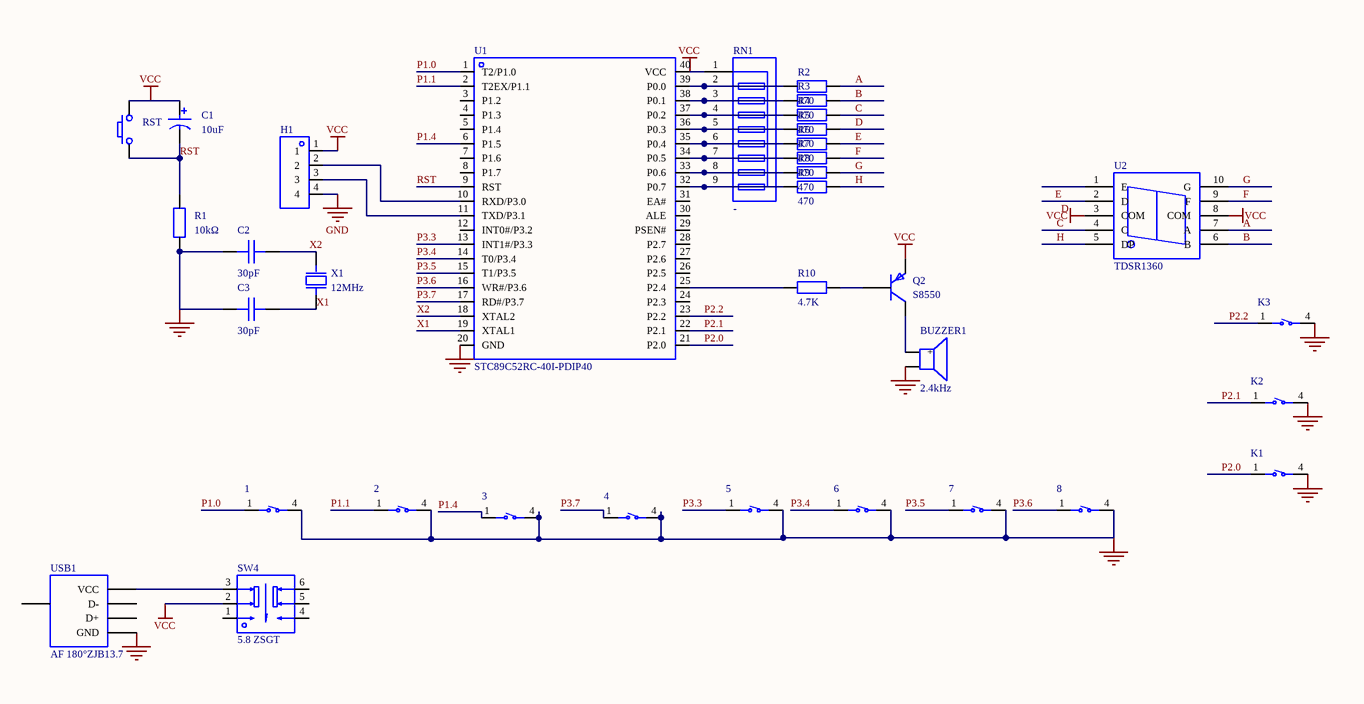
[diagram p0: MISC49928-3.schdoc]
# Altium project MISC49928-2.PrjPcb
1 sheet, 34 parts. Net scope: global (net labels, ports and power ports of the same name join across sheets).
Board file: MISC49928.pcbdoc

## Sheet MISC49928-3.schdoc
size 1187 x 839 mm; Version: V1.0; @Project Name: MISC49928; @Update Date: 2026-05-11; @Create Date: 2026-05-11; @Board Name: MISC49928; @Create Time: 23:58:54; @Page Count: 1; @Page No: 1; @Schematic Name: MISC49928; @Update Time: 23:58:54; Size: A4

### Parts
1  TS665CJ  [SW-TH_4P-L6.0-W6.0-P4.50-LS6.5]  (value not drawn)
2  TS665CJ  [SW-TH_4P-L6.0-W6.0-P4.50-LS6.5]  (value not drawn)
3  TS665CJ  [SW-TH_4P-L6.0-W6.0-P4.50-LS6.5]  (value not drawn)
4  TS665CJ  [SW-TH_4P-L6.0-W6.0-P4.50-LS6.5]  (value not drawn)
5  TS665CJ  [SW-TH_4P-L6.0-W6.0-P4.50-LS6.5]  (value not drawn)
6  TS665CJ  [SW-TH_4P-L6.0-W6.0-P4.50-LS6.5]  (value not drawn)
7  TS665CJ  [SW-TH_4P-L6.0-W6.0-P4.50-LS6.5]  (value not drawn)
8  TS665CJ  [SW-TH_4P-L6.0-W6.0-P4.50-LS6.5]  (value not drawn)
BUZZER1  2.4kHz  [BUZ-TH_BD12.0-P7.60-D0.6-FD]
C1  10uF  [CAP-TH_BD8.0-P3.50-D0.6-FD]
C2  30pF  [CAP-TH_L8.5-W5.0-P5.00-D1.2]
C3  30pF  [CAP-TH_L8.5-W5.0-P5.00-D1.2]
H1  (no value)  [HDR-TH_4P-P2.54-V-F]
K1  TS665CJ  [SW-TH_4P-L6.0-W6.0-P4.50-LS6.5]  (value not drawn)
K2  TS665CJ  [SW-TH_4P-L6.0-W6.0-P4.50-LS6.5]  (value not drawn)
K3  TS665CJ  [SW-TH_4P-L6.0-W6.0-P4.50-LS6.5]  (value not drawn)
Q2  S8550  [TO-92-3_L4.5-W3.5-P1.27-L]
R1  10kΩ  [RES-TH_BD2.4-L6.3-P10.30-D0.6]
R2  470  [R0603]
R3  470  [R0603]
R4  470  [R0603]
R5  470  [R0603]
R6  470  [R0603]
R7  470  [R0603]
R8  470  [R0603]
R9  470  [R0603]
R10  4.7K  [RES-TH_BD2.2-L6.5-P10.50-D0.6]
RN1  -  [RES-ARRAY-TH_9P-P2.54-D1.0]
RST  (no value)  [Key_TH_3.5x6x4.3]
SW4  5.8 ZSGT  [SW-TH_5.8ZSGT]
U1  STC89C52RC-40I-PDIP40  [DIP-40_L52.0-W13.7-P2.54-LS15.2-BL]
U2  TDSR1360  [LED-SEG-TH_10P-L17.6-W12.4-P2.54-S15.24-BL]
USB1  AF 180°ZJB13.7  [USB-A-TH_AF-ZJB13.7]
X1  12MHz  [HC-49US_L11.5-W4.5-P4.88]

### Nets
GND: 1.4(D) 2.4(D) 3.4(D) 4.4(D) 5.4(D) 6.4(D) 7.4(D) 8.4(D) BUZZER1.2 C2.1 C3.1 H1.4 K1.4(D) K2.4(D) K3.4(D) R1.1 U1.20(GND) USB1.4(GND)
VCC: C1.1 H1.1 Q2.1(E) RN1.1 RST.B SW4.2 U1.40(VCC) U2.3(COM) U2.8(COM)
A: R2.2 U2.7(A)
B: R3.2 U2.6(B)
C: R4.2 U2.4(C)
D: R5.2 U2.2(D)
E: R6.2 U2.1(E)
F: R7.2 U2.9(F)
G: R8.2 U2.10(G)
H: R9.2 U2.5(DP)
P1.0: 1.1(A) U1.1(T2/P1.0)
P1.1: 2.1(A) U1.2(T2EX/P1.1)
P1.4: 3.1(A) U1.6(P1.5)
P2.0: K1.1(A) U1.21(P2.0)
P2.1: K2.1(A) U1.22(P2.1)
P2.2: K3.1(A) U1.23(P2.2)
P3.3: 5.1(A) U1.13(INT1#/P3.3)
P3.4: 6.1(A) U1.14(T0/P3.4)
P3.5: 7.1(A) U1.15(T1/P3.5)
P3.6: 8.1(A) U1.16(WR#/P3.6)
P3.7: 4.1(A) U1.17(RD#/P3.7)
RST: C1.2 R1.2 RST.A U1.9(RST)
X1: C3.2 U1.19(XTAL1) X1.2(OSC2)
X2: C2.2 U1.18(XTAL2) X1.1(OSC1)
NetBUZZER1_1: BUZZER1.1(+) Q2.3(C)
NetH1_2: H1.2 U1.10(RXD/P3.0)
NetH1_3: H1.3 U1.11(TXD/P3.1)
NetQ2_2: Q2.2(B) R10.2
NetR2_1: R2.1 RN1.2 U1.39(P0.0)
NetR3_1: R3.1 RN1.3 U1.38(P0.1)
NetR4_1: R4.1 RN1.4 U1.37(P0.2)
NetR5_1: R5.1 RN1.5 U1.36(P0.3)
NetR6_1: R6.1 RN1.6 U1.35(P0.4)
NetR7_1: R7.1 RN1.7 U1.34(P0.5)
NetR8_1: R8.1 RN1.8 U1.33(P0.6)
NetR9_1: R9.1 RN1.9 U1.32(P0.7)
NetR10_1: R10.1 U1.25(P2.4)
NetSW4_3: SW4.3 USB1.1(VCC)

Not connected (* = marked no-connect by the designer): SW4 1 4 5 6; U1 3(P1.2) 4(P1.3) 5(P1.4) 7(P1.6) 8(P1.7) 12(INT0#/P3.2) 24(P2.3) 26(P2.5) 27(P2.6) 28(P2.7) 29(PSEN#) 30(ALE) 31(EA#); USB1 2(D-) 3(D+) 5(SHLD)

### Library data of the parts
1-8 K1-K3 = TS665CJ: Circuit structure: SPST; button shape: round button; actuating force: 2.5N; mounting: through-hole; switch length: 6mm; switch width: 6mm; switch height: 5mm; with bracket: no bracket; contact current: 50mA; rated voltage: 12V; with lamp: none; operating life: 5 ten-thousand cycles;; Manufacturer: SHOU HAN(首韩); AddInBom: yes; ModelId: 20eee248bc684ccd8cbdbb1d0d91ec6f0819f05c4eef4c71ace90d822a990e87; ModelName: SW-TH_4P-L6.0-W6.0-H5.0-LS6.5-P4.50; ModelTransform: 236.22,323.03,0,90,0,0,0,0,-137.795; Actuator/Cap Color: Black; Symbol: TS665CJ; Device: TS665CJ; LCSC Part Name: 6*6*5mm 直插 轻触开关; SupplierPart: C393938; ManufacturerPart: TS665CJ; Supplier Footprint: 插件-4P,6x6mm; JLCPCB Part Class: Extended Part; Datasheet: https://example.com/datasheet/TS665CJ/372550.html; Supplier: LCSC; ConvertToPcb: yes; FootprintName: SW-TH_4P-L6.0-W6.0-P4.50-LS6.5; Circuit: SPST; Actuator Style: Round button; Operating Force: 2.5N; Mounting Type: Through-hole; Length: 6mm; Width: 6mm; Switch Height: 5mm; with Bracket: No bracket; Contact Current: 50mA; Voltage Rating: 12V; With Lamp: None; Termination Style: PC pin; Life: 5 ten-thousand cycles; Operating Temperature: -25℃~+70℃
BUZZER1 = TMB12A05_C96093: Drive mode: active (built-in driver circuit); construction type: electromagnetic; rated voltage: 5V; frequency: 2.4kHz; sound pressure level (SPL): 85dB;; Manufacturer: 华能; AddInBom: yes; ModelId: 16ab50e14c5b4f2c986c135bdba60e370819f05c4eef4c71ace90d822a990e87; ModelName: BUZ-TH_D12.0-H9.5-P7.60; ModelTransform: 472.44,472.176,0,90,0,0,-0.787,0,-177.165; Voltage - Supply: 4V~8V; Current Consumption: 30mA; Symbol: TMB12A05; Device: TMB12A05_C96093; LCSC Part Name: 有源(内含驱动线路) 电磁式 2.4kHz; SupplierPart: C96093; ManufacturerPart: TMB12A05; Supplier Footprint: 插件,D=12mm; JLCPCB Part Class: Extended Part; Datasheet: https://example.com/datasheet/TMB12A05/97297.html; Supplier: LCSC; ConvertToPcb: yes; FootprintName: BUZ-TH_BD12.0-P7.60-D0.6-FD; Driver Circuitry: Active (built-in driver circuit); Technology: Electromagnetic; Voltage Rating: 5V; Value: 2.4kHz; Sound Pressure Level(SPL): 85dB; Diameter(φD): 12mm; Length: -; Width: -; Height: 9.8mm; Operating Temperature: -40℃~+85℃
C1 = ERK2GM100F12OT: Capacitance: 10uF; tolerance: ±20%; rated voltage: 400V; ripple current: 160mA@100kHz; equivalent series resistance (ESR): -;; Manufacturer: AISHI(艾华集团); AddInBom: yes; ModelId: a2c936ec27754f809f3966430e36f7670819f05c4eef4c71ace90d822a990e87; ModelName: CAP-TH_D8.0-H8.0-P3.50; ModelTransform: 314.96,314.862,0,180,0,0,0,0,-137.795; Pin Spacing: 3.5mm; Lifetime: 2000hrs@105℃; Symbol: ERK2GM100F12OT; Device: ERK2GM100F12OT; LCSC Part Name: 10uF ±20% 400V CLEAR 专门用于充电器; SupplierPart: C112497; ManufacturerPart: ERK2GM100F12OT; Supplier Footprint: 插件,D8xL12mm; JLCPCB Part Class: Extended Part; Datasheet: https://example.com/datasheet/ERK2GM100F12OT/113730.html; Supplier: LCSC; ConvertToPcb: yes; FootprintName: CAP-TH_BD8.0-P3.50-D0.6-FD; Value: 10uF; Tolerance: ±20%; Voltage Rating: 400V; Ripple Current: 160mA@100kHz; Equivalent Series Resistance(ESR): -; Diameter: 8mm; Height - Seated (Max): 12mm
C2 C3 = CC4-0805N300J500F3: Capacitance: 30pF; tolerance: ±5%; rated voltage: 50V; temperature coefficient: C0G;; Manufacturer: FH(风华); AddInBom: yes; ModelId: 5610b656e7164072960d9d2d8c7d4fdf0819f05c4eef4c71ace90d822a990e87; ModelName: CAP-TH_L4.2-W3.8-H3.8-P5.08; ModelTransform: 222.8342,149.606,0,0,0,0,0,0,-118.11; Symbol: CC4-0805N300J500F3; Device: CC4-0805N300J500F3; LCSC Part Name: 30pF ±5% 50V; SupplierPart: C94716; ManufacturerPart: CC4-0805N300J500F3; Supplier Footprint: 插件,P=5.08mm; JLCPCB Part Class: Extended Part; Datasheet: https://example.com/datasheet/CC4-0805N300J500F3/95914.html; Supplier: LCSC; ConvertToPcb: yes; FootprintName: CAP-TH_L8.5-W5.0-P5.00-D1.2; Value: 30pF; Tolerance: ±5%; Voltage Rating: 50V; Temperature Coefficient: C0G
H1 = HDR-F_2.54_1x4P: Symbol: 2.54-1*4P female; ConvertToPcb: yes; ModelId: d187812051054f85879fcaa51a310d8e0819f05c4eef4c71ace90d822a990e87; ModelTransform: 419.6842,98.464,0,0,0,0,0,0,-118.11; Device: HDR-F_2.54_1x4P; AddInBom: yes; SupplierPart: C2718488; Supplier Footprint: 插件; FootprintName: HDR-TH_4P-P2.54-V-F; ModelName: HDR-TH_4P-P2.54-V-F
Q2 = S8550_C2931493: Transistor type: PNP; collector current (Ic): 500mA; collector-emitter breakdown voltage (Vceo): 25V; power dissipation (Pd): 625mW; DC current gain (hFE): 160@50mA,1V;; Manufacturer: JSMSEMI(杰盛微); AddInBom: yes; ModelId: 45fa6cddef3743c6aacf8db740a3bc4c0819f05c4eef4c71ace90d822a990e87; ModelTransform: 177.165,137.795,0,0,0,0,0,29.528,-98.425; Transition frequency(fT): 150MHz; Current - Collector Cutoff: 100nA; Vce Saturation(VCE(sat)): 600mV@500mA,50mA; Emitter-Base Voltage(Vebo): 5V; Number: 1 PNP; Symbol: S8550_C2931493; Device: S8550_C2931493; LCSC Part Name: PNP 电流:500mA 电压:25V; SupplierPart: C2931493; ManufacturerPart: S8550; Supplier Footprint: TO-92; JLCPCB Part Class: Extended Part; Datasheet: https://example.com/datasheet/S8550/3272797.html; Supplier: LCSC; ConvertToPcb: yes; FootprintName: TO-92-3_L4.5-W3.5-P1.27-L; ModelName: TO-92-3_L4.5-W3.5-P1.27-L; type: PNP; Current - Collector(Ic): 500mA; Collector - Emitter Voltage VCEO: 25V; Pd - Power Dissipation: 625mW; DC Current Gain: 160@50mA,1V
R1 = MFR-25FTE52-10K: Resistor type: metal film resistor; resistance: 10kΩ; tolerance: ±1%; power: 250mW; temperature coefficient: ±50ppm/℃;; Manufacturer: YAGEO(国巨); AddInBom: yes; ModelId: 463263665006444ab7a47bd11b0cf9560819f05c4eef4c71ace90d822a990e87; ModelTransform: 427.165,94.32816,0,0,0,0,0,0,-196.85; Symbol: MFR-25FTE52-10K; Device: MFR-25FTE52-10K; LCSC Part Name: 金属膜电阻 10kΩ ±1% 250mW 铜脚，圆柱状直插; SupplierPart: C172967; ManufacturerPart: MFR-25FTE52-10K; Supplier Footprint: 插件,D2.4xL6.3mm; JLCPCB Part Class: Extended Part; Datasheet: https://example.com/datasheet/MFR-25FTE52-10K/184356.html; Supplier: LCSC; ConvertToPcb: yes; FootprintName: RES-TH_BD2.4-L6.3-P10.30-D0.6; ModelName: RES-TH_BD2.4-L6.3-P10.30-D0.6; Type: Metal film resistor; Value: 10kΩ; Tolerance: ±1%; Power(Watts): 250mW; Temperature Coefficient: ±50ppm/℃; Operating Temperature: -55℃~+155℃
R2-R9 = Res_0603: Symbol: Resistor; ConvertToPcb: yes; ModelId: fc143cca1e79419f9cd78b61e9279f080819f05c4eef4c71ace90d822a990e87; ModelTransform: 31.8897,63.7794,0,90,0,0,0,0,0; Device: Res_0603; Value: 470; AddInBom: yes; Supplier Footprint: 0603; FootprintName: R0603; ModelName: R0603
R10 = MFR0W4F4700A50: Resistor type: metal film resistor; resistance: 470Ω; tolerance: ±1%; power: 250mW; temperature coefficient: ±50ppm/℃;; Manufacturer: UNI-ROYAL(厚声); AddInBom: yes; ModelId: 259c3103781c424fb695c8049f0a17f30819f05c4eef4c71ace90d822a990e87; ModelTransform: 437.007,91.18383,0,0,0,0,0,0,-137.795; Voltage-Supply(Max): 250V; Symbol: MFR0W4F4700A50; Device: MFR0W4F4700A50; Value: 4.7K; LCSC Part Name: 470Ω ±1% 250mW 金属膜电阻 铜脚，圆柱状直插; ManufacturerPart: MFR0W4F4700A50; Supplier Footprint: 插件,D2.2xL6.5mm; JLCPCB Part Class: Extended Part; Datasheet: https://example.com/upload/public/pdf/source/20191012/C436293_8820AA14BC71FA35E551C06C441482A0.pdf; Supplier: LCSC; ConvertToPcb: yes; FootprintName: RES-TH_BD2.2-L6.5-P10.50-D0.6; ModelName: RES-TH_BD2.2-L6.5-P10.50-D0.6; Type: Metal film resistor; Tolerance: ±1%; Power(Watts): 250mW; Temperature Coefficient: ±50ppm/℃
RN1 = 排阻 10 K 5%: Number of resistors: -; resistance: -; power per element: -;; Symbol: 10 K 5%; Device: Resistor array 10 K 5%; 3D Model: d106c67f29e14d8080ba548247a719a10819f05c4eef4c71ace90d822a990e87; 3D Model Transform: 918.1084,118.11,0,0,0,0,0,0,-137.795; AddInBom: yes; ModelName: SIP-9_L22.8-W3.0-H8.5-P2.54; LCSC Part Name: 10KΩ (103) ±5%; Supplier Part: C26615; Manufacturer Part: 排阻 10 K 5%; Supplier Footprint: 插件; JLCPCB Part Class: Extended Part; Supplier: LCSC; Number of Resistors: -; Value: -; Power(Watts): -; Number of Pins: -; ConvertToPcb: yes; FootprintName: RES-ARRAY-TH_9P-P2.54-D1.0
RST = Key_TH_3.5x6x4.3: ConvertToPcb: yes; ModelId: c3523f9014d949d7ba5445190a3178990819f05c4eef4c71ace90d822a990e87; ModelName: SW-TH_L6.0-W3.5-H5.0-P6.5; ModelTransform: 308.49,137.8,335.08,0,0,0,0,0,-129.92; Symbol: Key_TH_3.5x6x4.3; Device: Key_TH_3.5x6x4.3; AddInBom: yes; Supplier Footprint: 插件; FootprintName: Key_TH_3.5x6x4.3
SW4 = 5.8 ZSGT: Circuit structure: DPDT; self-lock/no-lock: self-lock; mounting: through-hole; contact current: 110mA; rated voltage: 30V; with lamp: no; actuating force: 1.5N; operating life: 10 ten-thousand cycles;; Manufacturer: SHOU HAN(首韩); AddInBom: yes; ModelId: 3b6e980975cd43bda015b2e9aaa869d30819f05c4eef4c71ace90d822a990e87; ModelTransform: 228.346,228.346,0,0,0,0,0,0,-141.732; Actuator Style: Square button; Actuator/Cap Color: White; With Lamp: Without; Symbol: 5.8 ZSGT; Device: 5.8 ZSGT; LCSC Part Name: 5.8*5.8有头/高头 带锁/自锁开关 泡泡机开关; SupplierPart: C2681587; ManufacturerPart: 5.8 ZSGT; Supplier Footprint: 插件; JLCPCB Part Class: Extended Part; Datasheet: https://example.com/datasheet/5.8%2520ZSGT/2774930.html; Supplier: LCSC; ConvertToPcb: yes; FootprintName: SW-TH_5.8ZSGT; ModelName: SW-TH_5.8ZSGT; Circuit: DPDT; Self Lock / No Lock: Self-lock; Mounting Type: Through-hole; Contact Current: 110mA; Voltage Rating: 30V; Termination Style: PC pin; Operating Force: 1.5N; Operating Temperature: -10℃~+70℃; Life: 10 ten-thousand cycles
U1 = STC89C52RC-40I-PDIP40: CPU core: 51 family; CPU max frequency: -;; Manufacturer: STC; AddInBom: yes; ModelId: 16d4686a009b4ddca948f91eddb57b140819f05c4eef4c71ace90d822a990e87; ModelName: DIP-40_L52.3-W13.8-H4.0-LS15.24-P2.54; ModelTransform: 2059.051,615.743,0,0,0,0,0,0,-118.11; Program Storage Size: 8KB; Program Memory Type: FLASH; Voltage - Supply: 3.3V~5.5V; Symbol: STC89C52RC-40I; Device: STC89C52RC-40I-PDIP40; LCSC Part Name: 单片机原理及应用; SupplierPart: C14022; ManufacturerPart: STC89C52RC-40I-PDIP40; Supplier Footprint: DIP-40; JLCPCB Part Class: Extended Part; Datasheet: https://example.com/datasheet/STC89C52RC-40I-PDIP40/14679.html; Supplier: LCSC; ConvertToPcb: yes; FootprintName: DIP-40_L52.0-W13.7-P2.54-LS15.2-BL; CPU Core: 51 family; CPU Maximum Speed: -; RAM Size: -; EEPROM: -; Number of I/O: -; ADC (Bit): -; DAC (Bit): -
U2 = TDSR1360: Digits: 1; power dissipation (Pd): 185mW; emitting color: red; LED polarity: common cathode; digit/letter size (inch): 0.51;; Manufacturer: VISHAY(威世); AddInBom: yes; ModelId: 990eafc46e164274abc50912f2a6e67a0819f05c4eef4c71ace90d822a990e87; ModelTransform: 488.188,690.94358,0,0,0,0,0,0,-196.85; Number of Characters: 1 digit; Display Type: 7-segment; Digit/Alpha Size(inch): 0.51; Symbol: TDSR1360; Device: TDSR1360; LCSC Part Name: TDSR1360; SupplierPart: C5377595; ManufacturerPart: TDSR1360; Supplier Footprint: DIP-10; JLCPCB Part Class: Extended Part; Datasheet: https://example.com/datasheet/TDSR1360/6238758.html; Supplier: LCSC; ConvertToPcb: yes; FootprintName: LED-SEG-TH_10P-L17.6-W12.4-P2.54-S15.24-BL; ModelName: LED-SEG-TH_10P-L17.6-W12.4-P2.54-S15.24-BL; Size / Dimension: 17.5mmx12.25mmx6.4mm; Pd - Power Dissipation: 185mW; Illumination Color: Red; LED Polarity: Common cathode
USB1 = AF 180°ZJB13.7: Connector type: Type-A; standard: USB 2.0; gender: female; mounting: through-hole; contacts: 4P; ports: 1; rated current - power: 1.5A; operating temperature range: -25℃~+85℃;; Manufacturer: SHOU HAN(首韩); AddInBom: yes; ModelId: c3dea282a4a445c4ae65c8aa64bfab470819f05c4eef4c71ace90d822a990e87; ModelTransform: 562.991,271.653,0,0,0,0,0,3.78,-188.976; Number of Ports: 1; Rated Voltage (Max): 30V; Connect-Disconnect Life: 5 thousand cycles; Core Colour: White; Symbol: AF 180°ZJB13.7; Device: AF 180°ZJB13.7; LCSC Part Name: Type-A 母 直插; SupplierPart: C456015; ManufacturerPart: AF 180°ZJB13.7; Supplier Footprint: 插件; JLCPCB Part Class: Extended Part; Datasheet: https://example.com/upload/public/pdf/source/20241125/3F1287FBF237B0DC4F79F9BB9BA7EB30.pdf; Supplier: LCSC; ConvertToPcb: yes; FootprintName: USB-A-TH_AF-ZJB13.7; ModelName: USB-A-TH_AF-ZJB13.7; Connector Type: Type-A; Standard: USB 2.0; Gender: Female; Mounting Style: Through-hole; Number of Contacts: 4P; Current Rating - Power (Max): 1.5A; Supplementary Features: -; Center Height: -; Length: 13.7mm; Operating Temperature Range: -25℃~+85℃
X1 = X49SD12MSD2SC: Crystal type: through-hole crystal; frequency: 12MHz; normal temperature frequency deviation: ±20ppm; load capacitance: 20pF; frequency stability: ±30ppm;; Manufacturer: YXC(扬兴晶振); AddInBom: yes; ModelId: a8e34f6c394c4d60ace7720f62d1ccdf0819f05c4eef4c71ace90d822a990e87; ModelName: HC-49US_L11.0-W4.5-H3.5-P4.88; ModelTransform: 432.46488,177.165,0,0,0,0,0,0,-137.795; Symbol: X49SD12MSD2SC; Device: X49SD12MSD2SC; LCSC Part Name: HC-49US 12MHZ 20PF ±20PPM -20~70℃（±30PPM）; SupplierPart: C16369; ManufacturerPart: X49SD12MSD2SC; Supplier Footprint: HC-49S; JLCPCB Part Class: Extended Part; Datasheet: https://example.com/datasheet/X49SD12MSD2SC/17051.html; Supplier: LCSC; ConvertToPcb: yes; FootprintName: HC-49US_L11.5-W4.5-P4.88; Type: Through-hole crystal; Value: 12MHz; Normal temperature Frequency Tolerance: ±20ppm; Load Capacitance: 20pF; Frequency Stability: ±30ppm; Operating Temperature: -20℃~+70℃